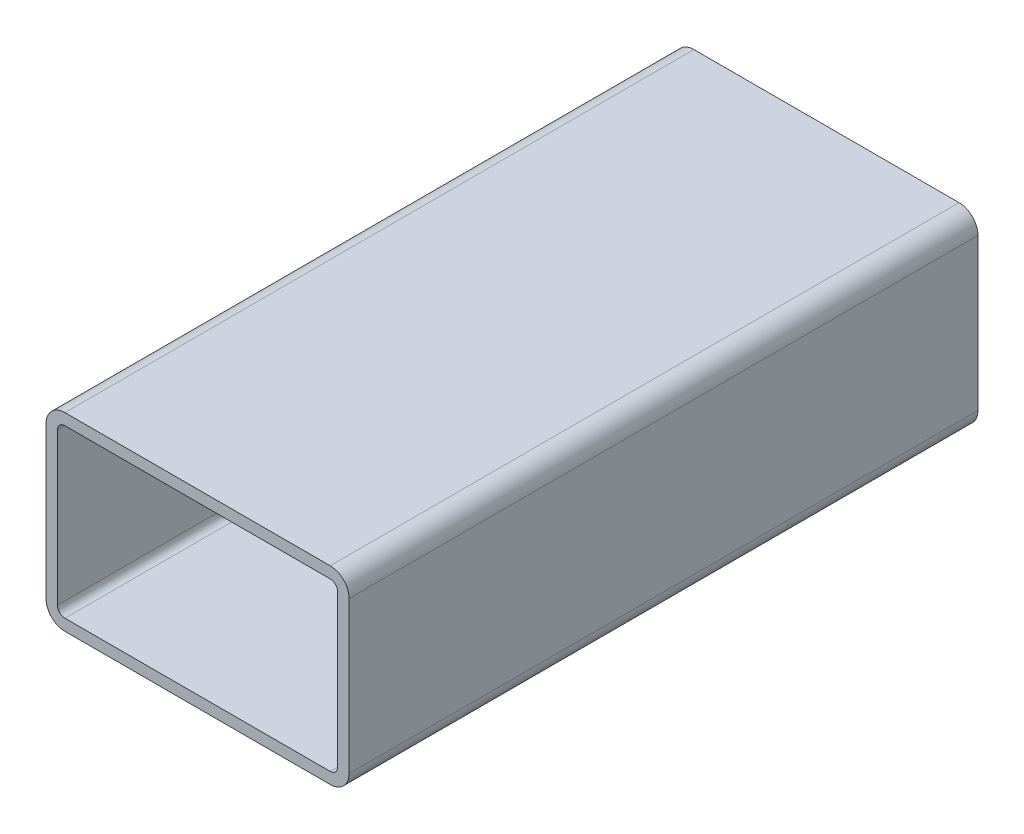
SolidWorks part; units mm, degrees
material "1023 Carbon Steel Plate (SS)"
ref_plane "Front Plane" through (0, 0, 0) normal (0, 0, 1) x (1, 0, 0)
ref_plane "Top Plane" through (0, 0, 0) normal (0, 1, 0) x (1, 0, 0)
ref_plane "Right Plane" through (0, 0, 0) normal (1, 0, 0) x (0, 0, -1)
sketch "Sketch1" plane through (0, 0, 0) normal (0, 0, 1) x (1, 0, 0)
  line L1 (40, 25) -> (-40, 25)
  line L2 (40, 25) -> (40, -25)
  line L3 (40, -25) -> (-40, -25)
  line L4 (-40, 25) -> (-40, -25)
  line L5 (40, 25) -> (-40, -25) construction
  line L6 (40, -25) -> (-40, 25) construction
  point P0 (0, 0)
  dimension "D1" = 80
  dimension "D2" = 50
extrude "Boss-Extrude1" add sketch "Sketch1" along normal blind 166
fillet "Fillet1" radius 5 4 edges at (40, -25, 83) (-40, -25, 83) (-40, 25, 83) (40, 25, 83)
shell "Shell1" thickness 3
